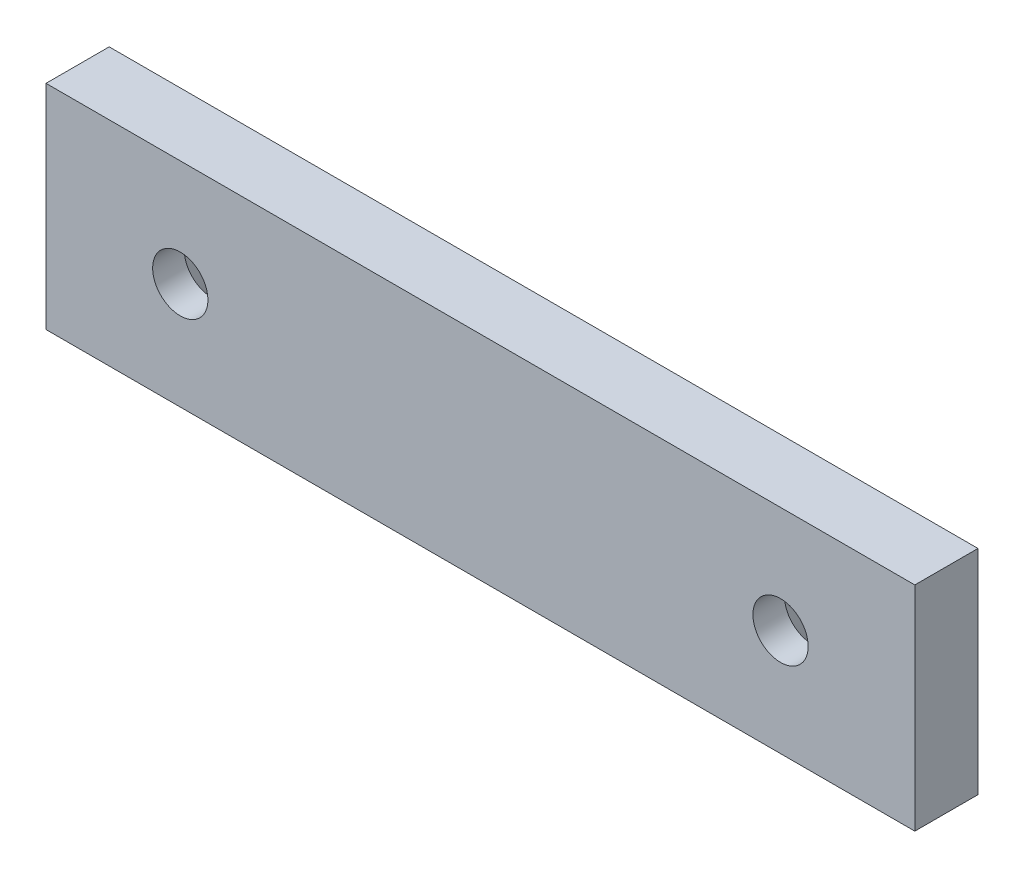
from build123d import *

# Parameters (mm, degrees)
SKETCH1_W           = 110
SKETCH1_H           = 27
BOSS_EXTRUDE1_DEPTH = 8


with BuildPart() as part:
    # Sketch1 → Boss-Extrude1 (new body)
    with BuildSketch(Plane.XY):
        Rectangle(SKETCH1_W, SKETCH1_H)
    extrude(amount=BOSS_EXTRUDE1_DEPTH)

    # Sketch2 → Cut-Revolve2 (revolve, cut)
    with BuildSketch(Plane(origin=(0, 0, 0), x_dir=(1, 0, 0), z_dir=(0, 1, 0)), mode=Mode.PRIVATE) as cut_revolve2_sk:
        Polygon((-30.5, 0), (-34.5, -4), (-34.5, -8), (-38, -8), (-38, 0), align=None)
    cut_revolve2 = revolve(cut_revolve2_sk.sketch.rotate(Axis((-38, 0, 0), (0, 0, 1)), 180), axis=Axis((-38, 0, 0), (0, 0, 1)), mode=Mode.SUBTRACT)

    # Mirror1: Cut-Revolve2 across plane
    add(cut_revolve2.mirror(Plane(origin=(0, 0, 0), x_dir=(0, 0, 1), z_dir=(1, 0, 0))), mode=Mode.SUBTRACT)


solid = part.part
